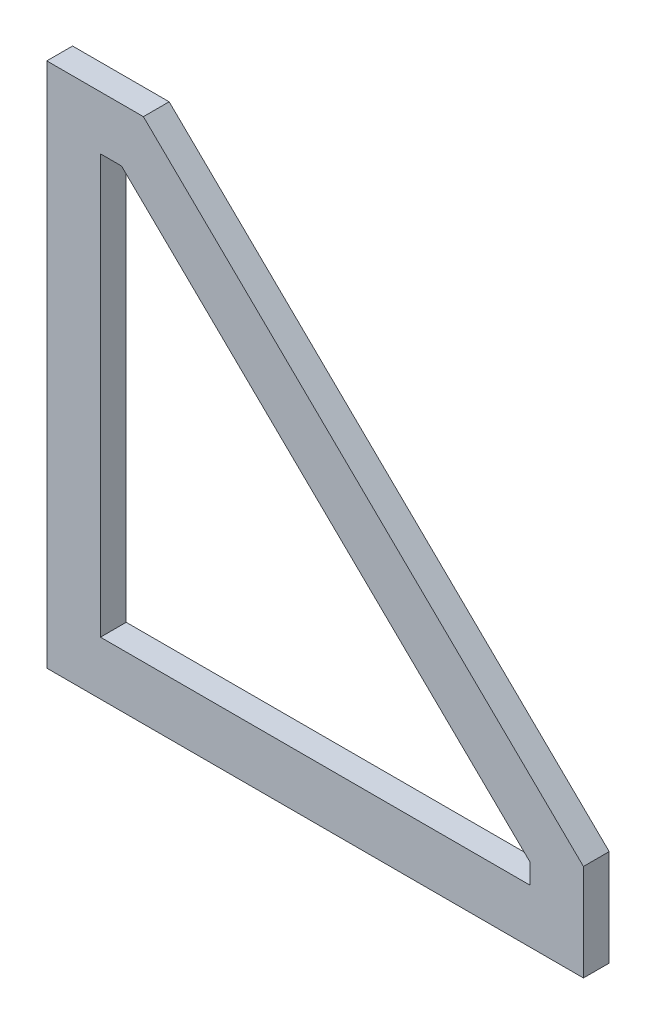
SolidWorks part; units mm, degrees
ref_plane "前视基准面" through (0, 0, 0) normal (0, 0, 1) x (1, 0, 0)
ref_plane "上视基准面" through (0, 0, 0) normal (0, 1, 0) x (1, 0, 0)
ref_plane "右视基准面" through (0, 0, 0) normal (1, 0, 0) x (0, 0, -1)
sketch "草图1" plane through (0, 0, 0) normal (0, 0, 1) x (1, 0, 0)
  line L0 (0, 0) -> (-250, 0)
  line L1 (-250, 0) -> (-250, 245)
  line L2 (-250, 245) -> (-205, 245)
  line L3 (-205, 245) -> (0, 45)
  line L4 (0, 45) -> (0, 0)
  line L5 (-225, 220) -> (-215.175, 220)
  line L6 (-215.175, 220) -> (-25, 34.4634)
  line L7 (-25, 34.4634) -> (-25, 25)
  line L8 (-25, 25) -> (-225, 25)
  line L9 (-225, 25) -> (-225, 220)
  dimension "D1" = 250
  dimension "D2" = 45
  dimension "D3" = 45
  dimension "D4" = 245
  dimension "D5" = 25
extrude "凸台-拉伸1" add sketch "草图1" along normal mid plane 12
